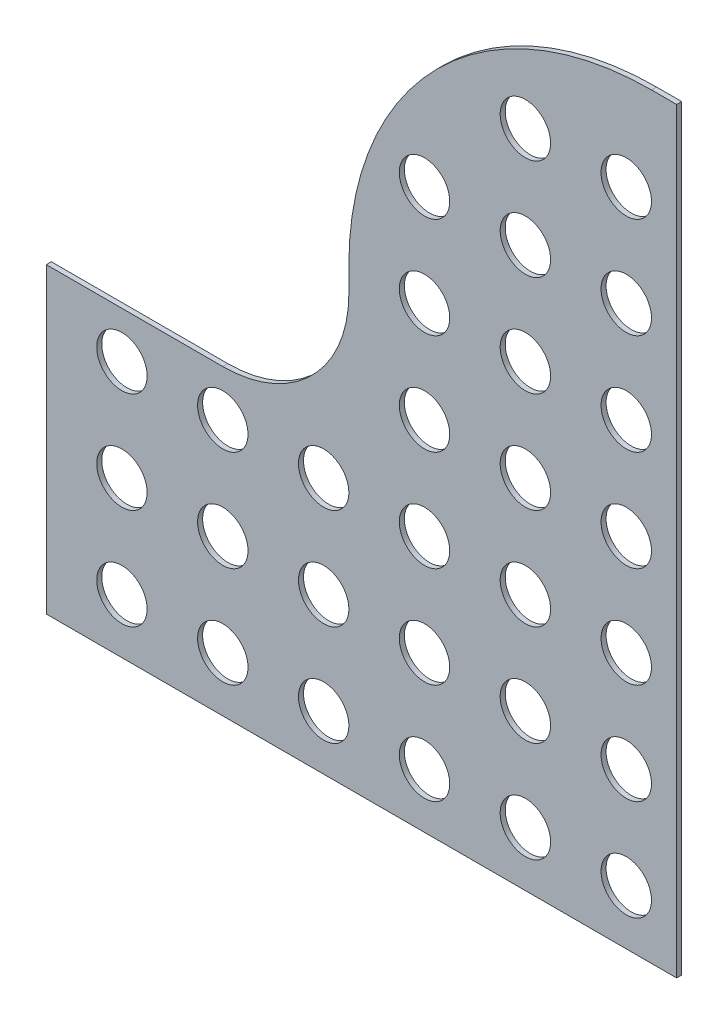
SolidWorks part; units mm, degrees
ref_plane "Front Plane" through (0, 0, 0) normal (0, 0, 1) x (1, 0, 0)
ref_plane "Top Plane" through (0, 0, 0) normal (0, 1, 0) x (1, 0, 0)
ref_plane "Right Plane" through (0, 0, 0) normal (1, 0, 0) x (0, 0, -1)
sketch "Sketch1" plane through (0, 0, 0) normal (0, 0, 1) x (1, 0, 0)
  line L0 (0, 0) -> (250, 0)
  line L1 (250, 0) -> (250, 300)
  line L2 (0, 0) -> (0, 120)
  line L3 (0, 120) -> (70, 120)
  line L5 (120, 170) -> (120, 180)
  line L6 (240, 300) -> (250, 300)
  arc A0 (120, 180) -> (240, 300) centre (240, 180) cw
  arc A1 (70, 120) -> (120, 170) centre (70, 170) ccw
  point P11 (120, 120)
  dimension "D5" = 120
  dimension "D6" = 50
  dimension "D1" = 120
  dimension "D2" = 250
  dimension "D3" = 300
  dimension "D4" = 120
extrude "Boss-Extrude1" add sketch "Sketch1" along normal blind 2
sketch "Sketch2" plane through (0, 0, 2) normal (0, 0, 1) x (1, 0, 0)
  line L0 (250, 0) -> (250, 300) construction
  circle A0 centre (230, 261.6988) radius 10
  circle A1 centre (190, 261.6988) radius 10
  circle A2 centre (230, 221.6988) radius 10
  circle A3 centre (190, 221.6988) radius 10
  circle A4 centre (230, 181.6988) radius 10
  circle A5 centre (190, 181.6988) radius 10
  circle A6 centre (230, 141.6988) radius 10
  circle A7 centre (190, 141.6988) radius 10
  circle A8 centre (230, 101.6988) radius 10
  circle A9 centre (190, 101.6988) radius 10
  circle A10 centre (230, 61.6988) radius 10
  circle A11 centre (190, 61.6988) radius 10
  circle A12 centre (230, 21.6988) radius 10
  circle A13 centre (190, 21.6988) radius 10
  circle A14 centre (150, 221.6988) radius 10
  circle A15 centre (150, 181.6988) radius 10
  circle A16 centre (150, 141.6988) radius 10
  circle A17 centre (150, 101.6988) radius 10
  circle A18 centre (150, 61.6988) radius 10
  circle A19 centre (150, 21.6988) radius 10
  circle A20 centre (110, 101.6988) radius 10
  circle A21 centre (70, 101.6988) radius 10
  circle A22 centre (30, 101.6988) radius 10
  circle A23 centre (110, 61.6988) radius 10
  circle A24 centre (70, 61.6988) radius 10
  circle A25 centre (30, 61.6988) radius 10
  circle A26 centre (110, 21.6988) radius 10
  circle A27 centre (70, 21.6988) radius 10
  circle A28 centre (30, 21.6988) radius 10
  dimension "D1" = 20
  dimension "D5" = 20
  dimension "D8" = 20
  dimension "D2" = 20
  dimension "D6" = 40
  dimension "D9" = 40
  dimension "D3" = 2
  dimension "D4" = 7
  dimension "D7" = 6
  dimension "D10" = 3
  dimension "D11" = 3
extrude "Cut-Extrude1" cut sketch "Sketch2" against normal blind 2
